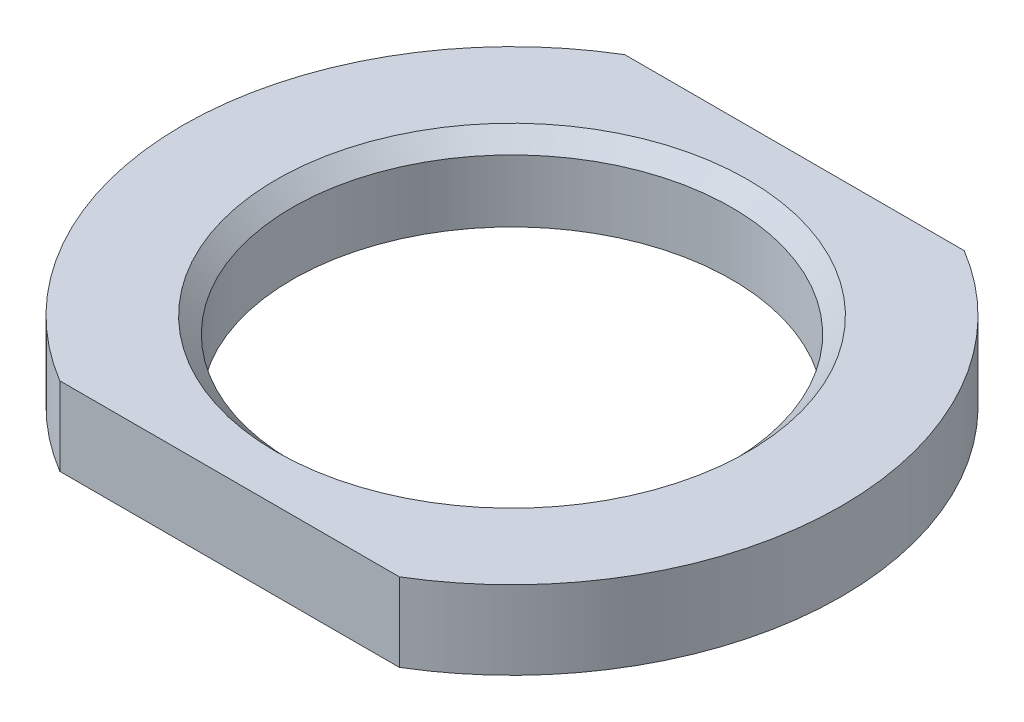
SolidWorks part; units mm, degrees
ref_plane "Front Plane" through (0, 0, 0) normal (0, 0, 1) x (1, 0, 0)
ref_plane "Top Plane" through (0, 0, 0) normal (0, 1, 0) x (1, 0, 0)
ref_plane "Right Plane" through (0, 0, 0) normal (1, 0, 0) x (0, 0, -1)
other "Configuration Table"
sketch "Sketch1" plane through (0, 0, 0) normal (0, 1, 0) x (1, 0, 0)
  line L0 (-10.8167, 18) -> (0, 18) construction
  line L1 (0, 18) -> (0, 0) construction
  line L2 (0, 0) -> (-37.3991, 0) construction
  line L3 (-10.8167, 18) -> (10.8167, 18)
  line L4 (-10.8167, -18) -> (10.8167, -18)
  circle A0 centre (0, 0) radius 21
  dimension "D1" = 42
  dimension "D2" = 18
extrude "Boss-Extrude1" add sketch "Sketch1" along normal blind 5 contours L4 A0 L3
hole_wizard "M30x2.0 Tapped Hole1" positions "Sketch2" profile "Sketch3" tap size "M30x2.0" standard "GB"
sketch "Sketch2" plane through (0, 5, 0) normal (0, 1, 0) x (1, 0, 0)
  point P0 (0, 0)
sketch "Sketch3" plane through (0, 5, 0) normal (1, 0, 0) x (0, 0, 1)
  line L0 (0, 0) -> (0, 78.412)
  line L1 (0, 78.412) -> (14, 70)
  line L2 (14, 70) -> (14, 1.025)
  line L3 (14, 1.025) -> (15.025, 0)
  line L5 (15.025, 0) -> (0, 0)
  line L6 (-14, 1.025) -> (-15.025, 0) construction
  line L10 (0, 78.412) -> (-14, 70) construction
  line L11 (0, -6.35) -> (0, 107.95) construction
  dimension "螺纹孔钻头直径" = 28
  dimension "螺纹孔钻头深度" = 70
  dimension "近端锥形沉头孔直径" = 30.05
  dimension "近端锥形沉头孔角度" = 90
  dimension "导头角度" = 118
cosmetic thread "Hole cosmetic thread1" parameters "D1"=60, "D2"=30
